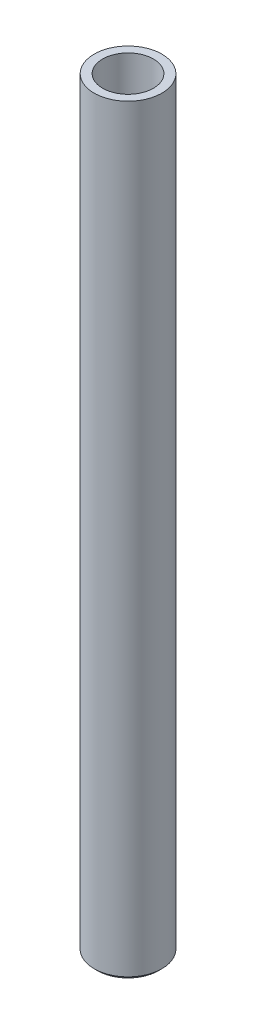
from build123d import *

# Parameters (mm, degrees)
SKETCH1_R           = 2
BOSS_EXTRUDE1_DEPTH = 45
CHAMFER1_SIZE       = 0.2
SKETCH3_R           = 1.5
CUT_EXTRUDE1_DEPTH  = 3


with BuildPart() as part:
    # Sketch1 → Boss-Extrude1 (new body)
    with BuildSketch(Plane(origin=(0, 0, 0), x_dir=(1, 0, 0), z_dir=(0, 1, 0))):
        with Locations(Location((0, 0, 0), (0, 0, 90))):
            Circle(SKETCH1_R)
    extrude(amount=BOSS_EXTRUDE1_DEPTH)

    # Chamfer1
    chamfer1_edges = [part.edges().sort_by_distance(p)[0] for p in [
        (0, 0, 2),
    ]]
    chamfer(chamfer1_edges, length=CHAMFER1_SIZE)

    # Sketch3 → Cut-Extrude1 (cut)
    with BuildSketch(Plane(origin=(0, 45, 0), x_dir=(1, 0, 0), z_dir=(0, 1, 0))):
        with Locations(Location((0, 0, 0), (0, 0, 270))):
            Circle(SKETCH3_R)
    extrude(amount=-CUT_EXTRUDE1_DEPTH, mode=Mode.SUBTRACT)


solid = part.part
